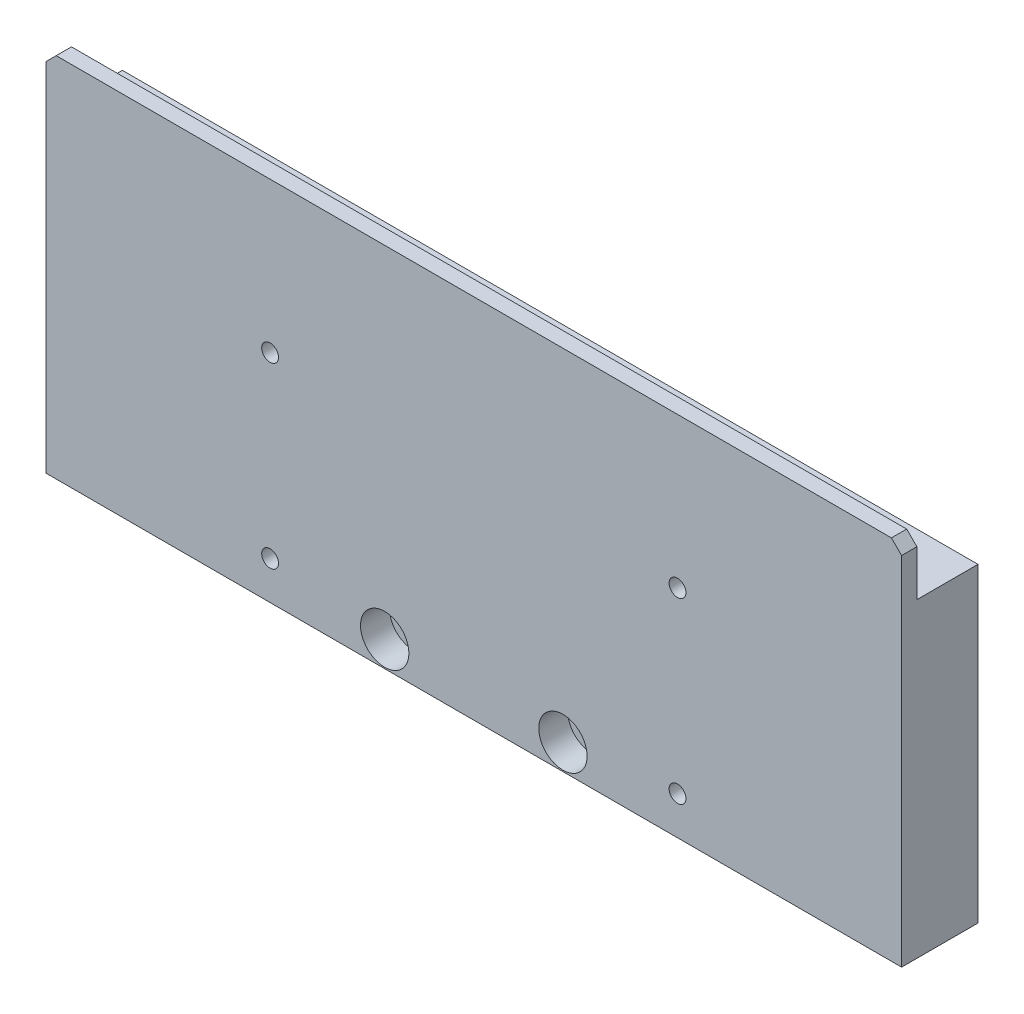
from build123d import *

# Parameters (mm, degrees)
BOSS_EXTRUDE1_DEPTH                                  = 7.5
SKETCH2_W                                            = 168
SKETCH2_H                                            = 12
CUT_EXTRUDE1_DEPTH                                   = 12
CUT_EXTRUDE2_DEPTH                                   = 489.185415595
SKETCH4_W                                            = 22
SKETCH4_H                                            = 220
CUT_EXTRUDE3_DEPTH                                   = 1.5
F_11_0_11_DIAMETER_HOLE1_D                           = 11
F_11_0_11_DIAMETER_HOLE1_DEPTH                       = 30
SKETCH17_W                                           = 13.5
SKETCH17_H                                           = 16
CUT_EXTRUDE4_DEPTH                                   = 5
M6_TAPPED_HOLE2_D                                    = 5
M6_TAPPED_HOLE2_DEPTH                                = 15
M6_TAPPED_HOLE2_TIP                                  = 1.502151548
M4_TAPPED_HOLE1_D                                    = 3.3
M4_TAPPED_HOLE1_DEPTH                                = 10.1
M4_TAPPED_HOLE1_TIP                                  = 0.991420021
HOLE_SIZE_PER_SOCKET_HEAD_CAP_SCREW_TYPE_D           = 11
HOLE_SIZE_PER_SOCKET_HEAD_CAP_SCREW_TYPE_CBORE_D     = 18
HOLE_SIZE_PER_SOCKET_HEAD_CAP_SCREW_TYPE_CBORE_DEPTH = 11
F_10_0_10_DIAMETER_HOLE1_D                           = 10
F_10_0_10_DIAMETER_HOLE1_DEPTH                       = 30
F_10_0_10_DIAMETER_HOLE1_TIP                         = 3.004303095
M8_TAPPED_HOLE3_D                                    = 6.8
M8_TAPPED_HOLE3_DEPTH                                = 19.75
M8_TAPPED_HOLE3_TIP                                  = 2.042926105
M6_TAPPED_HOLE3_D                                    = 5
M6_TAPPED_HOLE3_DEPTH                                = 15
M6_TAPPED_HOLE3_TIP                                  = 1.502151548
FILLET1_R                                            = 5
M5_TAPPED_HOLE1_D                                    = 4.2
M5_TAPPED_HOLE1_DEPTH                                = 12.4
M5_TAPPED_HOLE1_TIP                                  = 1.2618073
CHAMFER1_SIZE                                        = 1
SKETCH36_OUTSIDE_W                                   = 449.638
SKETCH36_OUTSIDE_H                                   = 439.638
SKETCH36_OUTSIDE_W_2                                 = 200
SKETCH36_OUTSIDE_H_2                                 = 72
CUT_EXTRUDE6_DEPTH                                   = 489.185415598
M4_TAPPED_HOLE2_D                                    = 3.3
M4_TAPPED_HOLE2_DEPTH                                = 10.1
M4_TAPPED_HOLE2_TIP                                  = 0.991420021
HOLE_SIZE_PER_SOCKET_HEAD_CAP_SCREW_2_D              = 5.5
HOLE_SIZE_PER_SOCKET_HEAD_CAP_SCREW_2_CBORE_D        = 9.5
HOLE_SIZE_PER_SOCKET_HEAD_CAP_SCREW_2_CBORE_DEPTH    = 5.7
CHAMFER2_SIZE                                        = 2


with BuildPart() as part:
    # Sketch1 → Boss-Extrude1 (new, symmetric)
    with BuildSketch(Plane.XY):
        Polygon((0, 0), (0, 340), (168, 340), (168, 220), (350, 220), (350, 0), align=None)
    extrude(amount=BOSS_EXTRUDE1_DEPTH, both=True)

    # Sketch2 → Cut-Extrude1 (cut)
    with BuildSketch(Plane(origin=(0, 340, 0), x_dir=(1, 0, 0), z_dir=(0, 1, 0))):
        with Locations((84, 1.5)):
            Rectangle(SKETCH2_W, SKETCH2_H)
    extrude(amount=-CUT_EXTRUDE1_DEPTH, mode=Mode.SUBTRACT)

    # Sketch3 → Cut-Extrude2 (cut, through all)
    with BuildSketch(Plane.XY.offset(7.5)):
        with BuildLine():
            Line((45, 110), (135, 110))
            ThreePointArc((135, 110), (138.535533906, 108.535533906), (140, 105))
            Line((140, 105), (140, 35))
            ThreePointArc((140, 35), (138.535533906, 31.464466094), (135, 30))
            Line((135, 30), (45, 30))
            ThreePointArc((45, 30), (41.464466094, 31.464466094), (40, 35))
            Line((40, 35), (40, 105))
            ThreePointArc((40, 105), (41.464466094, 108.535533906), (45, 110))
        make_face()
        with BuildLine():
            Line((215, 30), (305, 30))
            ThreePointArc((305, 30), (308.535533906, 31.464466094), (310, 35))
            Line((310, 35), (310, 105))
            ThreePointArc((310, 105), (308.535533906, 108.535533906), (305, 110))
            Line((305, 110), (215, 110))
            ThreePointArc((215, 110), (211.464466094, 108.535533906), (210, 105))
            Line((210, 105), (210, 35))
            ThreePointArc((210, 35), (211.464466094, 31.464466094), (215, 30))
        make_face()
    extrude(amount=-CUT_EXTRUDE2_DEPTH, mode=Mode.SUBTRACT)

    # Sketch4 → Cut-Extrude3 (cut)
    with BuildSketch(Plane(origin=(0, 0, -7.5), x_dir=(-1, 0, 0), z_dir=(0, 0, -1))):
        with Locations((-339, 110)):
            Rectangle(SKETCH4_W, SKETCH4_H)
    extrude(amount=-CUT_EXTRUDE3_DEPTH, mode=Mode.SUBTRACT)

    # Ø11.0 (11) Diameter Hole1
    with Locations(Plane(origin=(0, 30, 0), x_dir=(-1, 0, 0), z_dir=(0, 1, 0))):
        with Locations((-285, 0), (-65, 0), (-235, 0), (-115, 0)):
            Hole(F_11_0_11_DIAMETER_HOLE1_D / 2, depth=F_11_0_11_DIAMETER_HOLE1_DEPTH)

    # Sketch17 → Cut-Extrude4 (cut)
    with BuildSketch(Plane(origin=(350, 0, 0), x_dir=(0, 0, -1), z_dir=(1, 0, 0))):
        with Locations((-0.75, 160)):
            Rectangle(SKETCH17_W, SKETCH17_H)
    extrude(amount=-CUT_EXTRUDE4_DEPTH, mode=Mode.SUBTRACT)

    # M6 Tapped Hole2
    with Locations(Plane(origin=(0, 0, -7.5), x_dir=(-1, 0, 0), z_dir=(0, 0, -1))):
        with Locations((-290.5, 15), (-256.5, 15)):
            Hole(M6_TAPPED_HOLE2_D / 2, depth=M6_TAPPED_HOLE2_DEPTH)
            with Locations((0, 0, -(M6_TAPPED_HOLE2_DEPTH + M6_TAPPED_HOLE2_TIP / 2))):  # 118° drill point
                Cone(0, M6_TAPPED_HOLE2_D / 2, M6_TAPPED_HOLE2_TIP, mode=Mode.SUBTRACT)

    # M4 Tapped Hole1
    with Locations(Plane(origin=(0, 0, -6), x_dir=(-1, 0, 0), z_dir=(0, 0, -1))):
        with Locations((-335.5, 200), (-335.5, 140), (-335.5, 80), (-335.5, 20)):
            Hole(M4_TAPPED_HOLE1_D / 2, depth=M4_TAPPED_HOLE1_DEPTH)
            with Locations((0, 0, -(M4_TAPPED_HOLE1_DEPTH + M4_TAPPED_HOLE1_TIP / 2))):  # 118° drill point
                Cone(0, M4_TAPPED_HOLE1_D / 2, M4_TAPPED_HOLE1_TIP, mode=Mode.SUBTRACT)

    # Hole size per socket head cap screw type (through all)
    with Locations(Plane.XY.offset(7.5)):
        with Locations((70, 202), (100, 202), (130, 202), (130, 162), (100, 162), (70, 162)):
            CounterBoreHole(HOLE_SIZE_PER_SOCKET_HEAD_CAP_SCREW_TYPE_D / 2, HOLE_SIZE_PER_SOCKET_HEAD_CAP_SCREW_TYPE_CBORE_D / 2, HOLE_SIZE_PER_SOCKET_HEAD_CAP_SCREW_TYPE_CBORE_DEPTH)

    # Ø10.0 (10) Diameter Hole1
    with Locations(Plane.XY.offset(7.5)):
        with Locations((135, 135), (65, 135)):
            Hole(F_10_0_10_DIAMETER_HOLE1_D / 2, depth=F_10_0_10_DIAMETER_HOLE1_DEPTH)
            with Locations((0, 0, -(F_10_0_10_DIAMETER_HOLE1_DEPTH + F_10_0_10_DIAMETER_HOLE1_TIP / 2))):  # 118° drill point
                Cone(0, F_10_0_10_DIAMETER_HOLE1_D / 2, F_10_0_10_DIAMETER_HOLE1_TIP, mode=Mode.SUBTRACT)

    # M8 Tapped Hole3
    with Locations(Plane(origin=(350, 0, 0), x_dir=(0, 0, -1), z_dir=(1, 0, 0))):
        with Locations((0, 187.5), (0, 132.5)):
            Hole(M8_TAPPED_HOLE3_D / 2, depth=M8_TAPPED_HOLE3_DEPTH)
            with Locations((0, 0, -(M8_TAPPED_HOLE3_DEPTH + M8_TAPPED_HOLE3_TIP / 2))):  # 118° drill point
                Cone(0, M8_TAPPED_HOLE3_D / 2, M8_TAPPED_HOLE3_TIP, mode=Mode.SUBTRACT)

    # M6 Tapped Hole3
    with Locations(Plane(origin=(0, 328, 0), x_dir=(-1, 0, 0), z_dir=(0, 1, 0))):
        with Locations((-151.5, -1.5), (-106.5, -1.5), (-61.5, -1.5), (-16.5, -1.5)):
            Hole(M6_TAPPED_HOLE3_D / 2, depth=M6_TAPPED_HOLE3_DEPTH)
            with Locations((0, 0, -(M6_TAPPED_HOLE3_DEPTH + M6_TAPPED_HOLE3_TIP / 2))):  # 118° drill point
                Cone(0, M6_TAPPED_HOLE3_D / 2, M6_TAPPED_HOLE3_TIP, mode=Mode.SUBTRACT)

    # Fillet1
    fillet1_edges = [part.edges().sort_by_distance(p)[0] for p in [
        (168, 220, 0),
    ]]
    fillet(fillet1_edges, radius=FILLET1_R)

    # M5 Tapped Hole1
    with Locations(Plane(origin=(345, 0, 0), x_dir=(0, 0, -1), z_dir=(1, 0, 0))):
        with Locations((4, 160)):
            Hole(M5_TAPPED_HOLE1_D / 2, depth=M5_TAPPED_HOLE1_DEPTH)
            with Locations((0, 0, -(M5_TAPPED_HOLE1_DEPTH + M5_TAPPED_HOLE1_TIP / 2))):  # 118° drill point
                Cone(0, M5_TAPPED_HOLE1_D / 2, M5_TAPPED_HOLE1_TIP, mode=Mode.SUBTRACT)

    # Chamfer1
    chamfer1_edges = [part.edges().sort_by_distance(p)[0] for p in [
        (0, 0, 0),
        (0, 340, 6),
        (168, 340, 6),
        (350, 220, 0.75),
        (350, 0, 0.75),
    ]]
    chamfer(chamfer1_edges, length=CHAMFER1_SIZE)

    # Sketch36 outside → Cut-Extrude6 (cut, through all)
    with BuildSketch(Plane.XY.offset(7.5)):
        with Locations((175, 170)):
            Rectangle(SKETCH36_OUTSIDE_W, SKETCH36_OUTSIDE_H)
        with Locations((100, 303)):
            Rectangle(SKETCH36_OUTSIDE_W_2, SKETCH36_OUTSIDE_H_2, mode=Mode.SUBTRACT)
    extrude(amount=-CUT_EXTRUDE6_DEPTH, mode=Mode.SUBTRACT)

    # M4 Tapped Hole2
    with Locations(Plane.XY.offset(7.5)):
        with Locations((44, 309.5), (44, 274.5), (124, 274.5), (124, 309.5)):
            Hole(M4_TAPPED_HOLE2_D / 2, depth=M4_TAPPED_HOLE2_DEPTH)
            with Locations((0, 0, -(M4_TAPPED_HOLE2_DEPTH + M4_TAPPED_HOLE2_TIP / 2))):  # 118° drill point
                Cone(0, M4_TAPPED_HOLE2_D / 2, M4_TAPPED_HOLE2_TIP, mode=Mode.SUBTRACT)

    # Hole size per socket head cap screw  2 (through all)
    with Locations(Plane.XY.offset(7.5)):
        with Locations((66.5, 272), (101.5, 272)):
            CounterBoreHole(HOLE_SIZE_PER_SOCKET_HEAD_CAP_SCREW_2_D / 2, HOLE_SIZE_PER_SOCKET_HEAD_CAP_SCREW_2_CBORE_D / 2, HOLE_SIZE_PER_SOCKET_HEAD_CAP_SCREW_2_CBORE_DEPTH)

    # Chamfer2
    chamfer2_edges = [part.edges().sort_by_distance(p)[0] for p in [
        (168, 339, 6),
        (0, 339, 6),
    ]]
    chamfer(chamfer2_edges, length=CHAMFER2_SIZE)


solid = part.part
